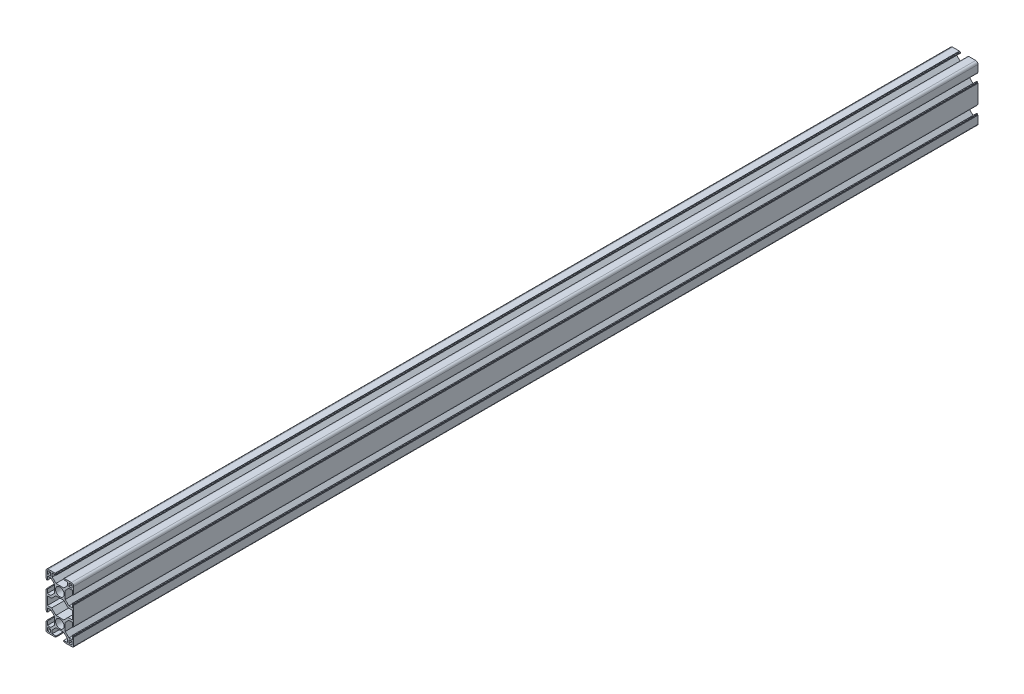
SolidWorks part; units mm, degrees
material "A6061 T6"
ref_plane "前视基准面" through (0, 0, 0) normal (0, 0, 1) x (1, 0, 0)
ref_plane "上视基准面" through (0, 0, 0) normal (0, 1, 0) x (1, 0, 0)
ref_plane "右视基准面" through (0, 0, 0) normal (1, 0, 0) x (0, 0, -1)
sketch "草图1" plane through (0, 0, 0) normal (0, 1, 0) x (1, 0, 0)
  line L0 (0, 0) -> (0, 980)
  dimension "D1" = 980
other "铝型材 30 X 60L X R2.5(1)"
ref_plane "基准面1" through (0, 0, 0) normal (0, 0, -1) x (-1, 0, 0)
sketch "Sketch1" plane through (0, 0, 0) normal (0, 0, -1) x (-1, 0, 0)
  line L0 (-5.1, 15) -> (-5.1, 14.5)
  line L1 (-5.1, 14.5) -> (-4.1, 14.5)
  line L2 (-4.1, 14.5) -> (-4.1, 13.5)
  line L3 (-4.1, 13.5) -> (-8.25, 13.5)
  line L4 (8.9, -10.45) -> (4.25, -5.8)
  line L5 (-15, -24.9) -> (-15, -5.1)
  line L6 (12.5, 15) -> (5.1, 15)
  line L7 (15, 12.5) -> (15, 5.1)
  line L8 (0, 15) -> (0, 0) construction
  line L9 (0, 0) -> (15, 0) construction
  line L10 (-8.25, 13.5) -> (-8.25, 9.8)
  line L11 (-8.25, 9.8) -> (-4.25, 5.8)
  line L12 (-4.25, 5.8) -> (4.25, 5.8)
  line L13 (8.25, 9.8) -> (4.25, 5.8)
  line L14 (8.25, 13.5) -> (8.25, 9.8)
  line L15 (4.1, 13.5) -> (8.25, 13.5)
  line L16 (4.1, 14.5) -> (4.1, 13.5)
  line L17 (5.1, 14.5) -> (4.1, 14.5)
  line L18 (5.1, 15) -> (5.1, 14.5)
  line L19 (-5.1, 15) -> (-12.5, 15)
  line L20 (15, 5.1) -> (14.5, 5.1)
  line L21 (14.5, 5.1) -> (14.5, 4.1)
  line L22 (14.5, 4.1) -> (13.5, 4.1)
  line L23 (13.5, 4.1) -> (13.5, 8.25)
  line L24 (13.5, 8.25) -> (9.8, 8.25)
  line L25 (9.8, 8.25) -> (5.8, 4.25)
  line L26 (5.8, 4.25) -> (5.8, -4.25)
  line L27 (9.8, -8.25) -> (5.8, -4.25)
  line L28 (13.5, -8.25) -> (9.8, -8.25)
  line L29 (13.5, -4.1) -> (13.5, -8.25)
  line L30 (14.5, -4.1) -> (13.5, -4.1)
  line L31 (14.5, -5.1) -> (14.5, -4.1)
  line L32 (15, -5.1) -> (14.5, -5.1)
  line L33 (8.9, -19.55) -> (4.25, -24.2)
  line L34 (-8.9, -19.55) -> (-4.25, -24.2)
  line L35 (-8.9, -10.45) -> (-4.25, -5.8)
  line L36 (-13.5, -10.45) -> (-8.9, -10.45)
  line L37 (-13.5, -19.55) -> (-8.9, -19.55)
  line L38 (-13.5, -10.45) -> (-9.8, -10.45) construction
  line L39 (4.25, -5.8) -> (-4.25, -5.8)
  line L40 (-13.5, -19.55) -> (-9.8, -19.55) construction
  line L41 (-13.5, -10.45) -> (-13.5, -19.55)
  line L42 (13.5, -10.45) -> (13.5, -19.55)
  line L43 (8.9, -10.45) -> (13.5, -10.45)
  line L44 (8.9, -19.55) -> (13.5, -19.55)
  line L45 (-11.625, 11.625) -> (-11.625, 16.245) construction
  line L46 (-15, -5.1) -> (-14.5, -5.1)
  line L47 (-14.5, -5.1) -> (-14.5, -4.1)
  line L48 (-14.5, -4.1) -> (-13.5, -4.1)
  line L49 (-13.5, -4.1) -> (-13.5, -8.25)
  line L50 (-13.5, -8.25) -> (-9.8, -8.25)
  line L51 (-9.8, -8.25) -> (-5.8, -4.25)
  line L52 (-5.8, -4.25) -> (-5.8, 4.25)
  line L53 (-9.8, 8.25) -> (-5.8, 4.25)
  line L54 (-13.5, 8.25) -> (-9.8, 8.25)
  line L55 (-13.5, 4.1) -> (-13.5, 8.25)
  line L56 (-14.5, 4.1) -> (-13.5, 4.1)
  line L57 (-14.5, 5.1) -> (-14.5, 4.1)
  line L58 (-15, 5.1) -> (-14.5, 5.1)
  line L59 (-13.375, 13.375) -> (-9.875, 13.375)
  line L60 (-15, 5.1) -> (-15, 12.5)
  line L61 (15, -5.1) -> (15, -24.9)
  line L62 (-13.375, 13.375) -> (-13.375, 9.875)
  line L63 (-13.375, 9.875) -> (-9.875, 9.875)
  line L64 (-9.875, 13.375) -> (-9.875, 9.875)
  line L65 (-11.625, 11.625) -> (-7.4229, 11.625) construction
  line L66 (-13.5, -45) -> (-5.1, -45)
  line L67 (-15, -43.5) -> (-15, -35.1)
  line L68 (9.875, 13.375) -> (13.375, 13.375)
  line L69 (9.875, 13.375) -> (9.875, 9.875)
  line L70 (9.875, 9.875) -> (13.375, 9.875)
  line L71 (13.375, 13.375) -> (13.375, 9.875)
  line L72 (-4.25, -24.2) -> (4.25, -24.2)
  line L73 (-13.375, -39.875) -> (-9.875, -39.875)
  line L74 (-13.375, -39.875) -> (-13.375, -43.375)
  line L75 (-13.375, -43.375) -> (-9.875, -43.375)
  line L76 (-9.875, -39.875) -> (-9.875, -43.375)
  line L77 (9.875, -39.875) -> (13.375, -39.875)
  line L78 (9.875, -39.875) -> (9.875, -43.375)
  line L79 (9.875, -43.375) -> (13.375, -43.375)
  line L80 (15, -24.9) -> (14.5, -24.9)
  line L81 (14.5, -24.9) -> (14.5, -25.9)
  line L82 (14.5, -25.9) -> (13.5, -25.9)
  line L83 (13.5, -25.9) -> (13.5, -21.75)
  line L84 (13.5, -21.75) -> (9.8, -21.75)
  line L85 (9.8, -21.75) -> (5.8, -25.75)
  line L86 (5.8, -25.75) -> (5.8, -34.25)
  line L87 (9.8, -38.25) -> (5.8, -34.25)
  line L88 (13.5, -38.25) -> (9.8, -38.25)
  line L89 (13.5, -34.1) -> (13.5, -38.25)
  line L90 (14.5, -34.1) -> (13.5, -34.1)
  line L91 (14.5, -35.1) -> (14.5, -34.1)
  line L92 (15, -35.1) -> (14.5, -35.1)
  line L93 (5.1, -45) -> (5.1, -44.5)
  line L94 (5.1, -44.5) -> (4.1, -44.5)
  line L95 (4.1, -44.5) -> (4.1, -43.5)
  line L96 (4.1, -43.5) -> (8.25, -43.5)
  line L97 (8.25, -43.5) -> (8.25, -39.8)
  line L98 (8.25, -39.8) -> (4.25, -35.8)
  line L99 (4.25, -35.8) -> (-4.25, -35.8)
  line L100 (-8.25, -39.8) -> (-4.25, -35.8)
  line L101 (-8.25, -43.5) -> (-8.25, -39.8)
  line L102 (-4.1, -43.5) -> (-8.25, -43.5)
  line L103 (-4.1, -44.5) -> (-4.1, -43.5)
  line L104 (-5.1, -44.5) -> (-4.1, -44.5)
  line L105 (-5.1, -45) -> (-5.1, -44.5)
  line L106 (-15, -35.1) -> (-14.5, -35.1)
  line L107 (-14.5, -35.1) -> (-14.5, -34.1)
  line L108 (-14.5, -34.1) -> (-13.5, -34.1)
  line L109 (-13.5, -34.1) -> (-13.5, -38.25)
  line L110 (-13.5, -38.25) -> (-9.8, -38.25)
  line L111 (-9.8, -38.25) -> (-5.8, -34.25)
  line L112 (-5.8, -34.25) -> (-5.8, -25.75)
  line L113 (-9.8, -21.75) -> (-5.8, -25.75)
  line L114 (-13.5, -21.75) -> (-9.8, -21.75)
  line L115 (-13.5, -25.9) -> (-13.5, -21.75)
  line L116 (-14.5, -25.9) -> (-13.5, -25.9)
  line L117 (-14.5, -24.9) -> (-14.5, -25.9)
  line L118 (-15, -24.9) -> (-14.5, -24.9)
  line L119 (5.1, -45) -> (13.5, -45)
  line L120 (13.375, -39.875) -> (13.375, -43.375)
  line L121 (15, -35.1) -> (15, -43.5)
  line L122 (0, -30) -> (15, -30) construction
  line L125 (5.1, -15) -> (5.1, -14.5) [skipped]
  line L127 (5.1, -14.5) -> (4.1, -14.5) [skipped]
  line L129 (4.1, -14.5) -> (4.1, -13.5) [skipped]
  line L131 (4.1, -13.5) -> (8.25, -13.5) [skipped]
  line L133 (-4.1, -13.5) -> (-8.25, -13.5) [skipped]
  line L135 (-4.1, -14.5) -> (-4.1, -13.5) [skipped]
  line L137 (-5.1, -14.5) -> (-4.1, -14.5) [skipped]
  line L139 (-5.1, -15) -> (-5.1, -14.5) [skipped]
  line L141 (-5.1, -15) -> (-5.1, -15.5) [skipped]
  line L142 (-5.1, -15.5) -> (-4.1, -15.5) [skipped]
  line L143 (-4.1, -15.5) -> (-4.1, -16.5) [skipped]
  line L144 (-4.1, -16.5) -> (-8.25, -16.5) [skipped]
  line L145 (12.5, -15) -> (5.1, -15) [skipped]
  line L146 (4.1, -16.5) -> (8.25, -16.5) [skipped]
  line L147 (4.1, -15.5) -> (4.1, -16.5) [skipped]
  line L148 (5.1, -15.5) -> (4.1, -15.5) [skipped]
  line L149 (5.1, -15) -> (5.1, -15.5) [skipped]
  line L150 (-5.1, -15) -> (-12.5, -15) [skipped]
  line L151 (-15, -24.9) -> (-15, -17.5) [skipped]
  line L152 (15, -17.5) -> (15, -24.9) [skipped]
  line L154 (-8.25, -13.5) -> (-8.25, -9.8) [skipped]
  line L156 (8.25, -13.5) -> (8.25, -9.8) [skipped]
  line L157 (8.25, -16.5) -> (8.25, -20.2) [skipped]
  line L158 (-8.25, -16.5) -> (-8.25, -20.2) [skipped]
  line L160 (-12.5, -14.05) -> (-9.7895, -11.3395) [skipped]
  line L161 (18.444, -10.006) -> (14.8, -13.65) [skipped]
  line L163 (11.9857, -13.5357) -> (9.7894, -11.3394) [skipped]
  line L164 (-15.9344, -12.5156) -> (-14.8, -13.65) [skipped]
  line L165 (9.7894, -15) -> (-9.8, -15) construction
  circle A0 centre (0, 0) radius 4.6
  arc A1 (-15, 12.5) -> (-12.5, 15) centre (-12.5, 12.5) cw
  arc A2 (15, 12.5) -> (12.5, 15) centre (12.5, 12.5) ccw
  arc A3 (15, -43.5) -> (13.5, -45) centre (13.5, -43.5) cw
  arc A4 (-15, -43.5) -> (-13.5, -45) centre (-13.5, -43.5) ccw
  circle A5 centre (0, -30) radius 4.6
  arc A12 (-15, -17.5) -> (-12.5, -15) centre (-12.5, -17.5) cw [skipped]
  arc A13 (15, -17.5) -> (12.5, -15) centre (12.5, -17.5) ccw [skipped]
  point P0 (-10, 0)
  point P1 (10, 0)
  point P2 (0, 20)
  point P4 (0, 0)
  point P5 (0, 0)
  point P6 (-10, 0)
  point P7 (15, 15)
  point P8 (-15, 15)
  point P12 (-15, -15)
  point P13 (15, -15)
  point P15 (0, -10)
  point P16 (10, 0)
  point P36 (-15, 15)
  point P39 (15, 15)
  point P43 (-10, -30)
  point P44 (10, -30)
  point P88 (0, -30)
  point P89 (0, -30)
  point P90 (-10, -30)
  point P91 (10, -30)
  point P102 (15, -45)
  point P120 (-15, -45)
  point P121 (0, 0)
  dimension "D1" = 16.5
  dimension "D2" = 30
  dimension "D3" = 8.2
  dimension "D4" = 10.2
  dimension "D5" = 9.2
  dimension "D6" = 9.2
  dimension "D7" = 2.5
  dimension "D8" = 45
  dimension "D14" = 30
  dimension "D15" = 1.5
  dimension "D9" = 0.5
  dimension "D10" = 1
  dimension "D11" = 8.5
  dimension "D12" = 15
  dimension "D13" = 60
  dimension "D16" = 45
  dimension "D17" = 45
  dimension "D18" = 10.2
  dimension "D19" = 8.2
  dimension "D20" = 2.2
  dimension "D22" = 3.5
  dimension "D21" = 2.2
